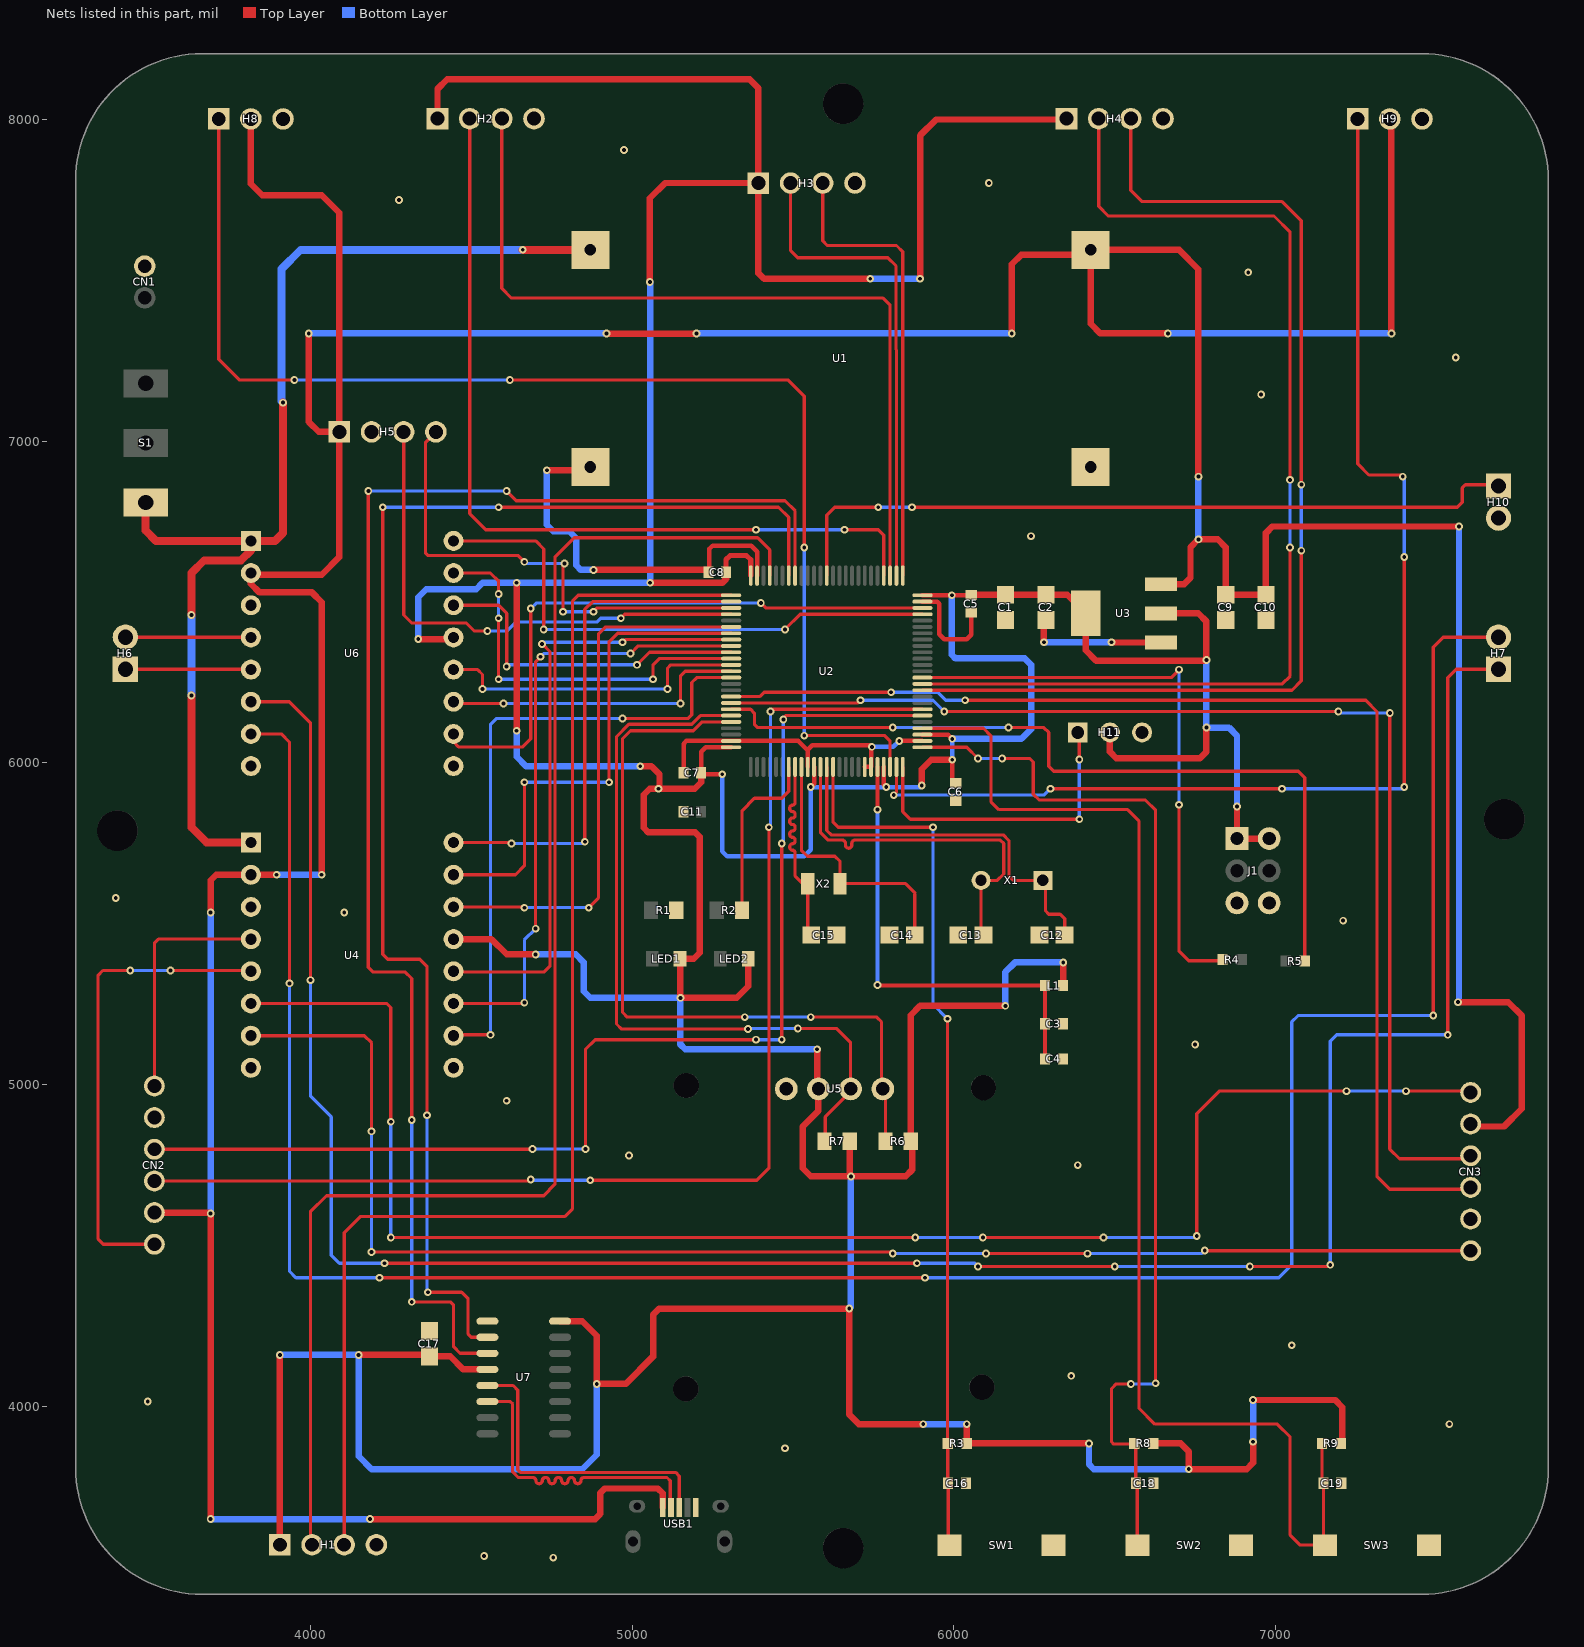
[diagram p0: the nets of this part, all layers, seen from the top]
# Altium PCB MISC62445.pcbdoc (part 2 of 3)
Units mil, origin at the board's own origin, x right, y up, seen from the top; angles counter-clockwise.
Board outline 4577.56 x 4789.41 mil, 2 copper layers (Top Layer, Bottom Layer), stack 62.206 mil thick; 68 components, 65 nets, 307 pads, 204 vias.

## Via types
v1: diameter 24.02, hole 12, Top Layer to Bottom Layer, 204 vias

## Nets (pads, with @x,y where several pads share a name; then routed paths per layer and width w, separated by ;. In a path a pad name is that pad's centre, name@x,y a point inside that pad or via, vN(x,y) a via of type N, cw(c..) or ccw(c..) an arc to the next point about the centre after c; other vN are vias at no path point) (continued)
+3.3V: C1.2 C2.2 C5.1 C6.1 C7.1 C8.1 C17.2 H1.1 H2.1 H3.1 H4.1 H11.2 J1.1 J1.2 L1.2 LED1.2 LED2.2 R3.2 R6.1 R7.1 R8.2 R9.2 U2.11 U2.22 U2.28 U2.50 U2.75 U2.100 U3.2 U3.4 U4.13 U5.2 U6.13 U7.4 U7.16 | length 23907.3
  Top Layer w14: C7.1@5214.56,5970 5214.56,6034.56 5228.78,6048.78 U2.100@5307.76,6048.78 ; C7.1@5215,5969.56 5219.56,5965 v1(5280,5965) ; v1(5555,5925) 5565.63,5935.63 U2.11@5565.63,5987.76 ; U2.22@5782.17,5987.76 5782.17,5932.83 v1(5790,5925) ; U2.28@5902.24,6088.15 5981.85,6088.15 v1(5995,6075) ; U2.50@5902.24,6521.22 v1(5993.7,6521.22) 6052.2,6521.22 C5.1@6053.62,6522.64 ; v1(5995,6010) 5995,5947.93 C6.1@6005.59,5937.33
  Top Layer w16: C8.1@5292.01,6593.37 5292.01,6632.01 5304.34,6644.34 5355.66,6644.34 5368.57,6631.43 U2.75@5368.57,6582.24
  Top Layer w20: H1.1@3905,3570 v1(3905,4160) ; v1(4150,4160) 4365.63,4160 C17.2@4370,4155.63 4434.37,4155.63 4475,4115 U7.4@4550.01,4115 ; v1(4335,6385) 4439.66,6385 U6.13@4444.92,6390.26 ; H2.1@4394.98,8002.56 4394.98,8094.98 4425,8125 5365,8125 5392.5,8097.5 H3.1@5392.5,7802.56 ; U4.13@4444.92,5452.44 4562.56,5452.44 4610,5405 v1(4700,5405) ; v1(4641.04,6100) v1(4641.04,6560) ; U7.16@4776.19,4265 4845,4265 4890,4220 v1(4890,4070) 4980,4070 5065,4155 5065,4285 5084.14,4304.14 v1(5675,4304.14) 5675,3975 5705,3945 v1(5905,3945) ; v1(5025,5990) 5060,5990 5085,5965 5085,5922.98 v1(5082.02,5920) ; v1(5055,7495) 5055,7755 5102.56,7802.56 H3.1@5392.5,7802.56 ; v1(5055.86,6560) 5056.19,6559.67 5279.67,6559.67 5292.01,6572.01 C8.1@5292.01,6593.37 ; C7.1@5214.56,5970 5215,5969.56 5215,5940 5195,5920 v1(5082.02,5920) ; LED2.2@5360.87,5391.41 5360.87,5305.87 5325,5270 v1(5150,5270) 5148.94,5271.06 LED1.2@5148.94,5391.41 5191.41,5391.41 5210,5410 5210,5770 5195.86,5784.14 5050,5784.14 5035.86,5798.28 5035.86,5900.86 5055,5920 v1(5082.02,5920) ; v1(5575,5110) 5575,4991.09 U5.2@5579.11,4986.98 5579.11,4919.11 5530,4870 5530,4740 5555,4715 v1(5680,4715) ; R7.1@5676.71,4824.66 5676.71,4718.29 v1(5680,4715) ; v1(5740,7505) 5410,7505 5392.5,7522.5 H3.1@5392.5,7802.56 ; v1(5895,7505) 5895,7950 5945,8000 6347.46,8000 H4.1@6350.02,8002.56 ; v1(5900,5930) 5900,5980 5930,6010 v1(5995,6010) ; v1(6040,3945) 6040,3885.13 R3.2@6040.13,3885 v1(6420,3885) ; C5.1@6053.62,6522.64 C1.2@6161.05,6522.64 C2.2@6286.5,6522.64 6352.49,6522.64 U3.4@6410.13,6465 6410.13,6349.87 6442.01,6317.99 6782.99,6317.99 v1(6785,6320) 6785,6440 6760,6465 U3.2@6643.98,6465 ; v1(6160,5245) 5895,5245 5866.06,5216.06 R6.1@5866.06,4824.66 5870,4820.73 5870,4735 5850,4715 v1(5680,4715) ; L1.2@6338.65,5307.86 6340,5309.21 v1(6340,5380) ; H11.2@6485,6095 6485,6035 6505,6015 6765,6015 6785,6035 v1(6785,6110) ; R8.2@6620,3885 6705,3885 6730,3860 v1(6730,3805) 6910,3805 6930,3825 v1(6930,3890) ; v1(6880,5865) J1.1@6880,5765 J1.2@6980,5765 ; v1(6930,4020) 7185,4020 7207.5,3997.5 7207.5,3889.13 R9.2@7203.37,3885
  Bottom Layer w14: v1(5280,5965) 5280,5725 5295,5710 5535,5710 5555,5730 v1(5555,5925) v1(5790,5925) 5895,5925 v1(5900,5930) ; v1(5995,6010) v1(5995,6075)
  Bottom Layer w20: v1(3905,4160) v1(4150,4160) 4150,3845 4190,3805 4845,3805 4890,3850 v1(4890,4070) ; v1(4335,6385) 4335,6515 4360,6540 4515,6540 4535,6560 v1(4641.04,6560) v1(5055.86,6560) 5055.86,7495.86 v1(5055,7495) ; v1(4641.04,6100) 4641.04,6018.96 4670,5990 v1(5025,5990) ; v1(4700,5405) 4825,5405 4850,5380 4850,5290 4870,5270 v1(5150,5270) 5150,5125 5165,5110 v1(5575,5110) ; v1(5675,4304.14) 5679.34,4308.49 5679.34,4714.34 v1(5680,4715) ; v1(5740,7505) v1(5895,7505) ; v1(5905,3945) v1(6040,3945) ; v1(5993.7,6521.22) 5993.7,6336.3 6005,6325 6220,6325 6240,6305 6240,6105 6210,6075 v1(5995,6075) ; v1(6160,5245) 6160,5350 6190,5380 v1(6340,5380) ; v1(6420,3885) 6420,3820 6435,3805 v1(6730,3805) ; v1(6785,6320) v1(6785,6110) 6855,6110 6880,6085 v1(6880,5865) ; v1(6930,3890) v1(6930,4020)
+5V: C9.2 C10.2 CN2.5 CN3.5 H5.1 H8.2 H9.2 U1.4 U3.3 U4.2 U6.2 USB1.1 | length 16715.7
  Top Layer w20: CN2.5@3515,4602.42 3687.58,4602.42 v1(3690,4600) v1(3690,3650) ; v1(3690,5535) 3690,5635 3707.44,5652.44 U4.2@3815,5652.44 v1(3895,5652.44) ; H8.2@3815,8001.77 3815,7800 3850,7765 4035,7765 4090,7710 H5.1@4090,7029.1 ; v1(3995,7335) 3995,7060 4025.9,7029.1 H5.1@4090,7029.1 ; v1(4035,5652.44) 4035,6500 4005,6530 3841.7,6530 3815,6556.7 U6.2@3815,6590.26 3820.26,6585 4035,6585 4090,6640 H5.1@4090,7029.1 ; v1(4185,3650) 4885,3650 4900.86,3665.86 4900.86,3730.86 4915,3745 5080,3745 5095.2,3729.8 USB1.1@5095.2,3686.2 ; v1(4920,7335) 4921.18,7333.82 5198.82,7333.82 v1(5200,7335) ; v1(6180,7335) 6180,7550 6210,7580 6410,7580 U1.4@6425,7595 ; U3.3@6643.98,6555.55 6715.55,6555.55 6735.55,6575.55 6735.55,6670.55 v1(6760,6695) 6820,6695 6845,6670 C9.2@6845,6522.64 C10.2@6970,6522.64 6970,6715 6990,6735 v1(7570,6735) ; v1(6665,7335) 6455,7335 6425,7365 U1.4@6425,7595 ; v1(6760,6890) 6760,7535 6700,7595 U1.4@6425,7595 ; H9.2@7355,8001.77 7360,7996.77 v1(7360,7335) ; v1(7566.64,5256.64) 7723.36,5256.64 7765,5215 7765,4925 7710,4870 7613.91,4870 CN3.5@7606.27,4877.64
  Bottom Layer w20: v1(3690,3650) v1(4185,3650) ; v1(3690,4600) v1(3690,5535) ; v1(3895,5652.44) v1(4035,5652.44) ; v1(3995,7335) v1(4920,7335) ; v1(5200,7335) v1(6180,7335) ; v1(6665,7335) v1(7360,7335) ; v1(6760,6695) v1(6760,6890) ; v1(7566.64,5256.64) 7570,5260 v1(7570,6735)
AL: CN2.3 U2.31 | length 3710
  Top Layer w10: CN2.3@3515,4799.27 4689.27,4799.27 v1(4690,4800) ; v1(4855,4800) 4855,5110 4885,5140 v1(5385,5140) ; v1(5465,5140) v1(5465,5750) ; v1(5470,6135) 5470,6140 5477.2,6147.2 U2.31@5902.24,6147.2
  Bottom Layer w10: v1(4690,4800) v1(4855,4800) ; v1(5385,5140) v1(5465,5140) ; v1(5465,5750) 5470,5755 v1(5470,6135)
AR: CN3.3 U2.92 | length 3793
  Top Layer w10: U2.92@5307.76,6206.26 5396.26,6206.26 5410,6220 v1(5805,6220) ; v1(6035,6195) 7280,6195 7315,6160 7315,4715 7355,4675 7600.48,4675 CN3.3@7606.27,4680.79
  Bottom Layer w10: v1(5805,6220) 5950,6220 5975,6195 v1(6035,6195)
BL: CN2.4 U2.32 | length 3825.1
  Top Layer w10: CN2.4@3515,4700.85 4680.85,4700.85 v1(4685,4705) ; v1(4870,4702.93) 5387.93,4702.93 5425,4740 v1(5425,5800) ; v1(5430,6160) 5436.89,6166.89 U2.32@5902.24,6166.89
  Bottom Layer w10: v1(4685,4705) 4687.07,4702.93 v1(4870,4702.93) ; v1(5425,5800) 5430,5805 v1(5430,6160)
BOOT0: R5.2 U2.94 | length 2523.3
  Top Layer w10: U2.94@5307.76,6166.89 5368.11,6166.89 5380,6155 5380,6120 5390,6110 v1(5810,6110) ; v1(6170,6110) 6280,6110 6295,6095 6295,5990 6310.6,5974.4 7070.6,5974.4 7090.6,5954.4 R5.2@7090.6,5383.95
  Bottom Layer w10: v1(5810,6110) v1(6170,6110)
BOOT1: R4.1 U2.37 | length 1832.4
  Top Layer w10: U2.37@5902.24,6265.32 6675.32,6265.32 v1(6700,6290) ; v1(6700,5870) 6700,5415 6730,5385 6831.39,5385 R4.1@6835.34,5388.95
  Bottom Layer w10: v1(6700,5870) v1(6700,6290)
BR: CN3.4 U2.93 | length 3689.8
  Top Layer w10: U2.93@5307.76,6186.57 5701.57,6186.57 v1(5710,6195) ; v1(5970,6160) v1(7195,6160) ; v1(7355,6155) 7355,4800 7385,4770 7597.06,4770 CN3.4@7606.27,4779.21
  Bottom Layer w10: v1(5710,6195) 5935,6195 v1(5970,6160) ; v1(7195,6160) 7200,6155 v1(7355,6155)
BT_RX: H5.4 U2.78 | length 1515.4
  Top Layer w10: H5.4@4390,7029.1 4357.93,6997.03 4357.93,6652.07 4365,6645 4645,6645 v1(4665,6625) ; v1(4785,6470) 4785,6615 v1(4790,6620) ; v1(4880,6470) 4891.85,6481.85 U2.78@5307.76,6481.85
  Bottom Layer w10: v1(4665,6625) 4670,6620 v1(4790,6620) ; v1(4785,6470) v1(4880,6470)
BT_TX: H5.3 U2.79 | length 1629.2
  Top Layer w10: H5.3@4290,7029.1 4290,6460 4315,6435 4485,6435 4510,6410 v1(4550,6410) ; v1(4965,6450) 4977.17,6462.17 U2.79@5307.76,6462.17
  Bottom Layer w10: v1(4550,6410) 4610,6410 4637.99,6437.99 4890.51,6437.99 4902.52,6450 v1(4965,6450)
ECHO_L: H2.3 U2.53 | length 2596.8
  Top Layer w10: H2.3@4594.98,8002.56 4594.98,7475.02 4625,7445 5780,7445 5801.85,7423.15 U2.53@5801.85,6582.24
ECHO_M: H3.3 U2.51 | length 1449.3
  Top Layer w10: H3.3@5592.5,7802.56 5592.5,7622.5 5606.71,7608.29 5821.71,7608.29 5841.22,7588.78 U2.51@5841.22,6582.24
ECHO_R: H4.3 U2.35 | length 3411.7
  Top Layer w10: U2.35@5902.24,6225.94 7050.94,6225.94 7080,6255 v1(7080,6660) ; H4.3@6550,8002.54 6550,7780 6585,7745 7020,7745 7080,7685 v1(7080,6865)
  Bottom Layer w10: v1(7080,6660) v1(7080,6865)
GND: C1.1 C2.1 C3.1 C4.1 C5.2 C6.2 C7.2 C8.2 C9.1 C10.1 C11.2 C12.1 C13.1 C14.1 C15.1 C16.1 C17.1 C18.1 C19.1 CN1.2 CN2.2 CN3.2 H1.4 H2.4 H3.4 H4.4 H5.2 H8.3 H9.3 H10.2 H11.3 J1.5 J1.6 R1.2 SW1.2 SW2.2 SW3.2 U1.2 U1.3 U2.10 U2.19 U2.20 U2.27 U2.49 U2.74 U2.99 U3.1 U4.3 U4.8 U4.9 U5.1 U6.3 U6.8 U6.9 U7.1 USB1.5 | length 2975.7
  Top Layer w14: C7.2@5159.44,5970 5160,5970.56 5160,6060 5168.46,6068.46 U2.99@5307.76,6068.46 5516.2,6068.46 5543.72,6040.94 5545.94,6040.94 ; C8.2@5240,6600.16 5240,6665.1 5249.9,6675 5370,6675 5388.46,6656.54 U2.74@5388.46,6582.24 ; U2.10@5545.94,5987.76 5545.94,6040.94 ; U2.19@5723.11,5987.76 U2.20@5742.8,5987.76 5742.8,6047.8 v1(5745,6050) 5740,6055 5560,6055 5545.94,6040.94 ; v1(5830,6068.46) U2.27@5902.24,6068.46 ; U2.49@5902.24,6501.54 5948.46,6501.54 5955,6495 5955,6400 5970,6385 6039.62,6385 6053.62,6399 C5.2@6053.62,6467.52
  Top Layer w20: v1(4735,6910) 4860,6910 U1.2@4870,6920 ; v1(4880,6600) C8.2@5230.26,6600 ; v1(6280,6375) 6280,6437.39 C2.1@6286.5,6443.9 ; v1(6490,6375) 6490.55,6374.45 U3.1@6643.98,6374.45
  Bottom Layer w14: v1(5745,6050) 5811.54,6050 v1(5830,6068.46)
  Bottom Layer w20: v1(4735,6910) 4735,6740 4755,6720 4804.49,6720 4825.86,6698.64 4825.86,6614.14 4840,6600 v1(4880,6600) ; v1(6280,6375) v1(6490,6375)
  other v1: 4755,3530 4540,3535 5475,3870 7540,3945 3494.28,4015 6365,4095 7050,4190 6385,4750 4990,4780 4610,4950 6750,5125 7210,5510 4105,5535 3395,5580 6240,6705 6955,7145 7560,7260 6915,7525 4275,7750 6108.73,7802.56 4975,7905
L+: H6.2 U6.4 | length 390.3
  Top Layer w10: H6.2@3425,6390.99 3814.27,6390.99 U6.4@3815,6390.26
L-: H6.1 U6.5 | length 390.3
  Top Layer w10: H6.1@3425,6290.99 3814.27,6290.99 U6.5@3815,6290.26
ML+: CN2.1 U4.4 | length 749
  Top Layer w10: CN2.1@3515,4996.12 3515,5440 3527.44,5452.44 U4.4@3815,5452.44
ML-: CN2.6 U4.5 | length 1483.9
  Top Layer w10: v1(3440,5355) 3355,5355 3340,5340 3340,4520 3356,4504 CN2.6@3515,4504 ; v1(3565,5355) 3812.44,5355 U4.5@3815,5352.44
  Bottom Layer w10: v1(3440,5355) v1(3565,5355)
MR+: CN3.1 U4.7 | length 4457.1
  Top Layer w10: U4.7@3815,5152.44 4167.56,5152.44 4190,5130 v1(4190,4855) ; v1(4190,4480) 5805,4480 v1(5810,4475) ; v1(6100,4475) v1(6415.05,4474.95) ; v1(6779.95,4484.95) 6780.96,4483.94 CN3.1@7606.27,4483.94
  Bottom Layer w10: v1(4190,4480) v1(4190,4855) ; v1(5810,4475) v1(6100,4475) ; v1(6415.05,4474.95) 6769.95,4474.95 v1(6779.95,4484.95)
MR-: CN3.6 U4.6 | length 4924.1
  Top Layer w10: U4.6@3815,5252.44 4237.56,5252.44 4250,5240 v1(4250,4885) ; v1(4250,4525) v1(5880,4525) ; v1(6090,4525) v1(6465,4525) ; v1(6755,4530) 6755,4910 6825,4980 v1(7220,4980) ; v1(7405,4980) 7602.33,4980 CN3.6@7606.27,4976.06
  Bottom Layer w10: v1(4250,4525) v1(4250,4885) ; v1(5880,4525) v1(6090,4525) ; v1(6465,4525) 6750,4525 v1(6755,4530) ; v1(7220,4980) v1(7405,4980)
OLED_SCL: R7.2 U2.95 U5.3 | length 2369.6
  Top Layer w10: U2.95@5307.76,6147.2 5212.2,6147.2 5185,6120 4990,6120 4951.44,6081.44 4951.44,5188.56 4967.07,5172.93 v1(5360,5172.93) ; v1(5515,5175) 5635,5175 5679.11,5130.89 U5.3@5679.11,4986.98 5679.11,4979.11 5600,4900 5600,4826.7 R7.2@5597.97,4824.66
  Bottom Layer w10: v1(5360,5172.93) 5362.07,5175 v1(5515,5175)
OLED_SDA: R6.2 U2.96 U5.4 | length 2402.4
  Top Layer w10: U2.96@5307.76,6127.52 5217.52,6127.52 5190,6100 4995,6100 4970,6075 4970,5225 4985,5210 v1(5350,5210) ; v1(5555,5210) 5760,5210 5775,5195 5775,4991.09 U5.4@5779.11,4986.98 5787.32,4978.77 R6.2@5787.32,4824.66
  Bottom Layer w10: v1(5350,5210) v1(5555,5210)
OSC32_IN: C15.2 U2.8 X2.2 | length 623.5
  Top Layer w10: U2.8@5506.57,5987.76 5506.57,5877.16 cw(c5498.28,5877.16) 5498.28,5868.88 ccw(c5498.28,5860.59) 5490,5860.59 5490,5857.16 ccw(c5498.28,5857.16) 5498.28,5848.88 cw(c5498.28,5840.59) 5506.57,5840.59 5506.57,5837.16 cw(c5498.28,5837.16) 5498.28,5828.88 ccw(c5498.28,5820.59) 5490,5820.59 5490,5817.16 ccw(c5498.28,5817.16) 5498.28,5808.88 cw(c5498.28,5800.59) 5506.57,5800.59 5506.57,5797.16 cw(c5498.28,5797.16) 5498.28,5788.88 ccw(c5498.28,5780.59) 5490,5780.59 5490,5777.16 ccw(c5498.28,5777.16) 5498.28,5768.88 cw(c5498.28,5760.59) 5506.57,5760.59 5506.57,5757.16 cw(c5498.28,5757.16) 5498.28,5748.88 ccw(c5498.28,5740.59) 5490,5740.59 5490,5737.16 ccw(c5498.28,5737.16) 5498.28,5728.88 cw(c5498.28,5720.59) 5506.57,5720.59 5506.57,5648.43 5530,5625 X2.2@5545.86,5625 ; X2.2@5545.86,5620 5545.86,5475.83 C15.2@5556.69,5465
OSC32_OUT: C14.2 U2.9 X2.1 | length 832.8
  Top Layer w10: U2.9@5526.26,5987.76 5526.26,5728.74 5545,5710 5630,5710 5646.26,5693.74 X2.1@5646.26,5625 5850,5625 5878.53,5596.47 ; C14.2@5878.53,5465 5878.53,5591.47
OSC_IN: C13.2 U2.12 X1.2 | length 1167.7
  Top Layer w10: U2.12@5585.32,5987.76 5585.32,5784.68 5609.69,5760.31 5652.87,5760.31 cw(c5652.87,5750.31) 5662.87,5750.31 5662.87,5745 ccw(c5672.87,5745) 5682.87,5745 5682.87,5750.31 cw(c5692.87,5750.31) 5692.87,5760.31 6144.69,5760.31 6155,5750 6155,5655 6135,5635 6084.45,5635 6084.45,5472.86 C13.2@6092.32,5465
OSC_OUT: C12.2 U2.13 X1.1 | length 1216.6
  Top Layer w10: U2.13@5605,5987.76 5605,5790 5618.69,5776.31 6153.69,5776.31 6171,5759 6171,5649 6185,5635 X1.1@6276.58,5635 6285,5626.57 6285,5540 6295,5530 6330,5530 6344.37,5515.63 C12.2@6344.37,5465
PA0: H8.1 U2.23 | length 4023.6
  Top Layer w10: H8.1@3715,8001.77 3715,7255 3780,7190 v1(3950,7190) ; v1(4620,7190) 5485,7190 5535,7140 v1(5535,6670) ; v1(5535,6085) 5785,6085 5801.85,6068.15 U2.23@5801.85,5987.76
  Bottom Layer w10: v1(3950,7190) v1(4620,7190) ; v1(5535,6085) v1(5535,6670)
PA1: H9.1 U2.24 | length 3883.7
  Top Layer w10: v1(5813.23,5900) 5821.54,5908.31 U2.24@5821.54,5987.76 ; v1(6300,5920) v1(7020,5920) ; H9.1@7255,8001.77 7255,6930 7290,6895 7390,6895 v1(7395,6890) ; v1(7400,5925) v1(7400,6640)
  Bottom Layer w10: v1(5813.23,5900) 6280,5900 v1(6300,5920) ; v1(7020,5920) 7395,5920 v1(7400,5925) ; v1(7395,6890) 7400,6885 v1(7400,6640)
PA2: H11.1 U2.25 | length 969.7
  Top Layer w10: U2.25@5841.22,5987.76 5841.22,5848.78 5865,5825 v1(6390,5825) ; H11.1@6385,6095 6390,6090 v1(6390,6010.92)
  Bottom Layer w10: v1(6390,5825) v1(6390,6010.92)
PA3: C18.2 R8.1 SW2.1 U2.26 | length 3349.1
  Top Layer w10: U2.26@5902.24,6048.78 6040,6048.78 v1(6075,6013.78) ; v1(6150,6013.78) 6236.22,6013.78 6246.93,6003.07 6246.93,5903.07 6265,5885 6595,5885 6627.07,5852.93 v1(6627.07,4072.07) ; v1(6550,4070) 6505,4070 6490,4055 6490,3890 6497.07,3882.93 6558.61,3882.93 R8.1@6560.68,3885 6565.59,3880.1 C18.2@6565.59,3761.54 6570.21,3756.91 SW2.1@6570.21,3568.9
  Bottom Layer w10: v1(6075,6013.78) v1(6150,6013.78) ; v1(6550,4070) 6625,4070 v1(6627.07,4072.07)
PA4: C19.2 R9.1 SW3.1 U2.29 | length 3990.9
  Top Layer w10: U2.29@5902.24,6107.83 6092.17,6107.83 6115,6085 6115,5880 6140,5855 6540,5855 6575,5820 6575,3995 6625,3945 7005,3945 7045,3905 7045,3600 7076.1,3568.9 SW3.1@7153.58,3568.9 7148.95,3573.53 C19.2@7148.95,3761.54 7144.05,3766.44 R9.1@7144.05,3885
PA9: U2.68 U7.3 | length 4565.2
  Top Layer w10: v1(4180,6845) 4180,5365 4195,5350 4295,5350 4315,5330 v1(4315,4890) ; v1(4315,4325) 4435,4325 4445,4315 4445,4185 4465,4165 U7.3@4550.01,4165 ; v1(4610,6845) 4640,6815 5475,6815 5506.57,6783.43 U2.68@5506.57,6582.24
  Bottom Layer w10: v1(4180,6845) v1(4610,6845) ; v1(4315,4325) v1(4315,4890)
PA10: U2.69 U7.2 | length 4320
  Top Layer w10: v1(4225,6795) 4225,5405 4240,5390 4340,5390 4362.07,5367.93 v1(4362.07,4905) ; v1(4365,4355) 4470,4355 4490,4335 4490,4225 4500,4215 U7.2@4550.01,4215 ; v1(4585,6795) 5455,6795 5486.89,6763.11 U2.69@5486.89,6582.24
  Bottom Layer w10: v1(4225,6795) v1(4585,6795) ; v1(4362.07,4905) 4362.07,4357.93 v1(4365,4355)
PA13: H1.2 U2.72 | length 4570.6
  Top Layer w10: H1.2@4005,3570 4000,3575 4000,4605 4050,4655 4725,4655 4760,4690 4760,6640 4820,6700 5390,6700 5427.83,6662.17 U2.72@5427.83,6582.24
PA14: H1.3 U2.76 | length 4099.7
  Top Layer w10: H1.3@4105,3570 4105,4540 4155,4590 4790,4590 4815,4615 4815,6503.56 4832.66,6521.22 U2.76@5307.76,6521.22
PA15: U2.77 U4.16 | length 1598.2
  Top Layer w10: U4.16@4444.92,5752.44 4622.56,5752.44 v1(4625,5750) ; v1(4852.93,5755) 4852.93,6477.24 4877.23,6501.54 U2.77@5307.76,6501.54
  Bottom Layer w10: v1(4625,5750) 4847.93,5750 v1(4852.93,5755)
PB1: H4.2 U2.36 | length 3433.5
  Top Layer w10: U2.36@5902.24,6245.63 7020.63,6245.63 7045,6270 v1(7045,6670) ; H4.2@6450.02,8002.56 6450.02,7730 6480.02,7700 6995,7700 7045,7650 v1(7045,6880)
  Bottom Layer w10: v1(7045,6670) v1(7045,6880)
PB3: U2.89 U4.10 | length 1947.7
  Top Layer w10: U4.10@4444.92,5152.44 4447.48,5155 v1(4560,5155) ; v1(4970,6137.93) 5172.93,6137.93 5185,6150 5185,6250 5200.32,6265.32 U2.89@5307.76,6265.32
  Bottom Layer w10: v1(4560,5155) 4560,6120 4577.93,6137.93 v1(4970,6137.93)
PB10: U2.47 U6.16 | length 1737.3
  Top Layer w10: U6.16@4444.92,6690.26 4699.74,6690.26 4725,6665 v1(4725,6415) ; v1(5475,6415) 5522.17,6462.17 U2.47@5902.24,6462.17
  Bottom Layer w10: v1(4725,6415) v1(5475,6415)
PB11: U2.48 U6.10 | length 1917.4
  Top Layer w10: U6.10@4444.92,6090.26 4444.92,6065.08 4460,6050 4660,6050 4685,6075 v1(4685,6480) ; v1(5400,6497.01) 5415.16,6481.85 U2.48@5902.24,6481.85
  Bottom Layer w10: v1(4685,6480) 4702.01,6497.01 v1(5400,6497.01)
PB13: H3.2 U2.52 | length 1520.6
  Top Layer w10: H3.2@5492.5,7802.56 5492.5,7592.5 5515,7570 5795,7570 5820,7545 5820,7285 5821.54,7283.46 U2.52@5821.54,6582.24
PB15: H2.2 U2.54 | length 2668.1
  Top Layer w10: H2.2@4494.98,8002.56 4494.98,6775.02 4545,6725 v1(5385,6725) ; v1(5660,6725) 5765,6725 5782.17,6707.83 U2.54@5782.17,6582.24
  Bottom Layer w10: v1(5385,6725) v1(5660,6725)
PC6: H10.1 U2.63 | length 2343
  Top Layer w10: U2.63@5605,6582.24 5605,6770 5630,6795 v1(5765,6795) ; v1(5870,6795) 7565,6795 7580,6810 7580,6855 7590,6865 7688.78,6865 H10.1@7692.83,6860.94
  Bottom Layer w10: v1(5765,6795) v1(5870,6795)
PC13: R2.2 U2.7 | length 556.1
  Top Layer w10: R2.2@5341.59,5541.61 5341.59,5851.59 5380,5890 5465,5890 5486.89,5911.89 U2.7@5486.89,5987.76
PD0: U2.81 U4.14 | length 1706.6
  Top Layer w10: U4.14@4444.92,5552.44 4662.56,5552.44 v1(4665,5550) ; v1(4865,5550) 4895,5580 4895,6400 4917.8,6422.8 U2.81@5307.76,6422.8
  Bottom Layer w10: v1(4665,5550) 4666.02,5551.02 4863.98,5551.02 v1(4865,5550)
PD1: U2.82 U4.15 | length 1581.8
  Top Layer w10: U4.15@4444.92,5652.44 4637.44,5652.44 4665,5680 v1(4665,5940) ; v1(4928.44,5940) 4928.44,6376.56 4955,6403.11 U2.82@5307.76,6403.11
  Bottom Layer w10: v1(4665,5940) v1(4928.44,5940)
PD2: U2.83 U4.12 | length 1913.1
  Top Layer w10: U4.12@4444.92,5352.44 4447.36,5350 4725,5350 4745,5370 4745,6345 v1(4720,6370) ; v1(4970,6375) 4978.43,6383.43 U2.83@5307.76,6383.43
  Bottom Layer w10: v1(4720,6370) 4725,6375 v1(4970,6375)
PD3: U2.84 U4.11 | length 1923.6
  Top Layer w10: U4.11@4444.92,5252.44 4662.44,5252.44 v1(4665,5255) ; v1(4700,5485) 4700,6315 v1(4715,6330) ; v1(4995,6340) 5018.74,6363.74 U2.84@5307.76,6363.74
  Bottom Layer w10: v1(4665,5255) 4665,5450 v1(4700,5485) ; v1(4715,6330) 4725,6340 v1(4995,6340)
PD4: U2.85 U6.14 | length 1056.6
  Top Layer w10: U6.14@4444.92,6490.26 4584.74,6490.26 4610,6465 v1(4610,6300) ; v1(5015,6305) 5054.06,6344.06 U2.85@5307.76,6344.06
  Bottom Layer w10: v1(4610,6300) 4615,6305 v1(5015,6305)
PD5: U2.86 U6.15 | length 1231.3
  Top Layer w10: U6.15@4444.92,6590.26 4559.74,6590.26 4585,6565 v1(4585,6525) ; v1(4585,6260) v1(4585,6450) ; v1(5065,6260) 5065,6305 5084.37,6324.37 U2.86@5307.76,6324.37
  Bottom Layer w10: v1(4585,6260) v1(5065,6260) ; v1(4585,6450) v1(4585,6525)
PD6: U2.87 U6.12 | length 983.2
  Top Layer w10: U6.12@4444.92,6290.26 4519.74,6290.26 4535,6275 v1(4535,6230) ; v1(5110,6230) 5110,6295 5119.69,6304.69 U2.87@5307.76,6304.69
  Bottom Layer w10: v1(4535,6230) v1(5110,6230)
PD7: U2.88 U6.11 | length 956.2
  Top Layer w10: U6.11@4444.92,6190.26 4450.18,6185 v1(4600,6185) ; v1(5150,6185) 5150,6270 5165,6285 U2.88@5307.76,6285
  Bottom Layer w10: v1(4600,6185) v1(5150,6185)
R+: H7.2 U6.7 | length 7479.3
  Top Layer w10: U6.7@3815,6090.26 3909.74,6090.26 3935,6065 v1(3935,5315) ; v1(4215,4400) v1(5910,4400) ; v1(7490,5215) 7490,6360 7520.99,6390.99 H7.2@7692.83,6390.99
  Bottom Layer w10: v1(3935,5315) 3935,4420 3955,4400 v1(4215,4400) ; v1(5910,4400) 7010,4400 7050,4440 7050,5195 7070,5215 v1(7490,5215)
R-: H7.1 U6.6 | length 7362.4
  Top Layer w10: U6.6@3815,6190.26 3934.74,6190.26 4000,6125 v1(4000,5325) ; v1(4230,4445) v1(5885,4445) ; v1(6075,4435) v1(6500,4435) ; v1(6920,4435) 7165,4435 v1(7170,4440) ; v1(7535,5155) 7535,6265 7560.99,6290.99 H7.1@7692.83,6290.99
  Bottom Layer w10: v1(4000,5325) 4000,4965 4065,4900 4065,4470 4090,4445 v1(4230,4445) ; v1(5885,4445) 6065,4445 v1(6075,4435) ; v1(6500,4435) v1(6920,4435) ; v1(7170,4440) 7170,5135 7190,5155 v1(7535,5155)
RST: C16.2 R3.1 SW1.1 U2.14 | length 2742.7
  Top Layer w10: U2.14@5624.69,5987.76 5624.69,5815.31 5640,5800 v1(5935,5800) ; R3.1@5977.32,3885 R3.1@5978.9,3886.51 ; R3.1@5980,3885.81 v1(5980,5205) ; R3.1@5980.81,3885 5980.81,3762.95 C16.2@5982.22,3761.54 5982.22,3573.53 SW1.1@5986.85,3568.9
  Bottom Layer w10: v1(5935,5800) 5935,5250 v1(5980,5205)
USBD+: U7.5 USB1.3 | length 955.3
  Top Layer w10: U7.5@4550.01,4065 4630,4065 4644.43,4050.57 4644.43,3803.19 4652.63,3795 5135,3795 5146.4,3783.6 USB1.3@5146.4,3686.2
USBD-: U7.6 USB1.2 | length 961.6
  Top Layer w10: U7.6@4550.01,4015 4621.36,4015 4628.43,4007.93 4628.43,3796.57 4646,3779 4691.3,3779 cw(c4691.3,3769.5) 4700.8,3769.5 ccw(c4710.3,3769.5) 4710.3,3760 4711.3,3760 ccw(c4711.3,3769.5) 4720.8,3769.5 cw(c4730.3,3769.5) 4730.3,3779 4731.3,3779 cw(c4731.3,3769.5) 4740.8,3769.5 ccw(c4750.3,3769.5) 4750.3,3760 4751.3,3760 ccw(c4751.3,3769.5) 4760.8,3769.5 cw(c4770.3,3769.5) 4770.3,3779 4771.3,3779 cw(c4771.3,3769.5) 4780.8,3769.5 ccw(c4790.3,3769.5) 4790.3,3760 4791.3,3760 ccw(c4791.3,3769.5) 4800.8,3769.5 cw(c4810.3,3769.5) 4810.3,3779 4811.3,3779 cw(c4811.3,3769.5) 4820.8,3769.5 ccw(c4830.3,3769.5) 4830.3,3760 4831.3,3760 ccw(c4831.3,3769.5) 4840.8,3769.5 cw(c4850.3,3769.5) 4850.3,3779 5108.37,3779 5118.69,3768.69 USB1.2@5118.69,3688.31
VM: S1.1 U1.1 U4.1 U6.1 | length 3584
  Top Layer w25: S1.1@3487.96,6810 3487.96,6722.04 3519.74,6690.26 U6.1@3815,6690.26 ; v1(3630,6210) 3630,5800 3677.56,5752.44 U4.1@3815,5752.44 ; v1(3630,6460) 3630,6590 3670,6630 3784.76,6630 3815,6660.24 U6.1@3815,6690.26 ; v1(3915,7120) 3915,6715.26 3890,6690.26 U6.1@3815,6690.26 ; v1(4660,7595) U1.1@4870,7595
  Bottom Layer w25: v1(3630,6210) v1(3630,6460) ; v1(3915,7120) 3910,7125 3910,7535 3970,7595 v1(4660,7595)
VREF+: C3.2 C4.2 L1.1 U2.21 | length 1427.6
  Top Layer w13: v1(5762.48,5310) 5764.62,5307.86 L1.1@6283.54,5307.86 C3.2@6283.53,5190 C4.2@6283.53,5080 ; v1(5762.48,5855) U2.21@5762.48,5987.76
  Bottom Layer w13: v1(5762.48,5310) v1(5762.48,5855)
pads on no net: S1.3 SCREW1.1 SCREW2.1 SCREW3.1 SCREW4.1 SCREW5.1 SCREW6.1 SCREW7.1 SCREW8.1 U2.1 U2.2 U2.3 U2.4 U2.5 U2.15 U2.16 U2.17 U2.18 U2.30 U2.33 U2.34 U2.38 U2.39 U2.40 U2.41 U2.42 U2.43 U2.44 U2.45 U2.46 U2.55 U2.56 U2.57 U2.58 U2.59 U2.60 U2.61 U2.62 U2.64 U2.65 U2.66 U2.67 U2.70 U2.71 U2.73 U2.80 U2.90 U2.91 U2.97 U2.98 U7.7 U7.8 U7.9 U7.10 U7.11 U7.12 U7.13 U7.14 U7.15 USB1.4 USB1.6 USB1.7 USB1.8 USB1.9

## Polygon pours and split planes (outlines as drawn)
GND on Top Layer (solid, remove dead copper, pour order 0): 3155,8360 3155,3265 8030,3265 8030,8360
GND on Bottom Layer (solid, remove dead copper, pour order 2): 3000,8540 3000,3000 8340,3000 8340,8540

## Keep-outs
Board Outline Layer:
  the board outline again, w10

## Other copper
Top Layer:
  drawing of 339 lines, arcs and shapes, not listed
Bottom Layer:
  drawing of 182 lines, arcs and shapes, not listed